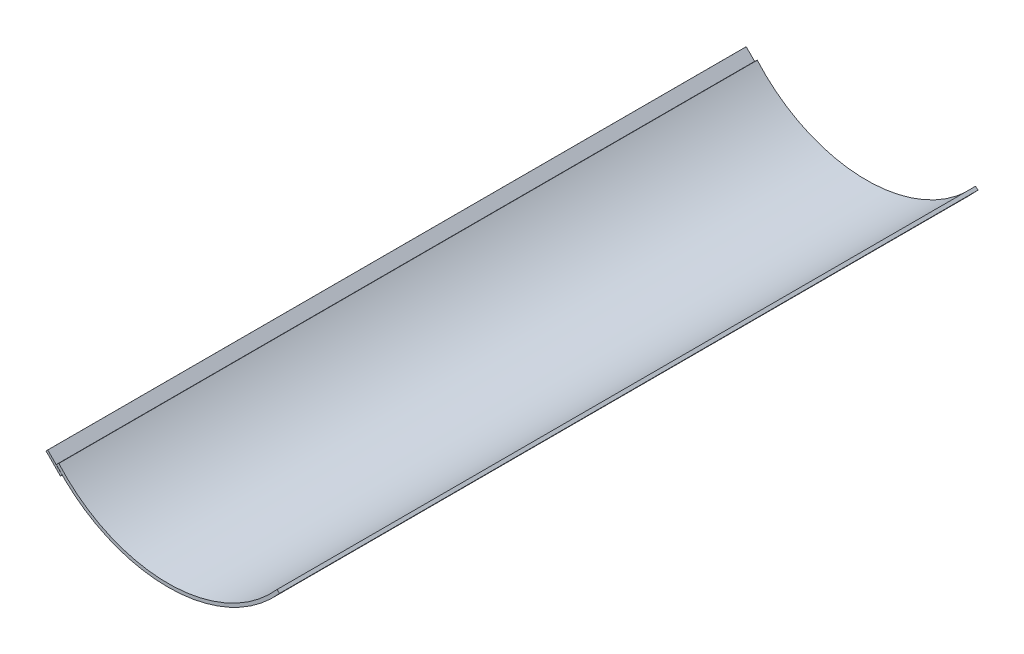
SolidWorks part; units mm, degrees
material "Q235A"
ref_plane "前视基准面" through (0, 0, 0) normal (0, 0, 1) x (1, 0, 0)
ref_plane "上视基准面" through (0, 0, 0) normal (0, 1, 0) x (1, 0, 0)
ref_plane "右视基准面" through (0, 0, 0) normal (1, 0, 0) x (0, 0, -1)
sketch "草图1" plane through (0, 0, 0) normal (0, 0, 1) x (1, 0, 0)
  line L0 (-132.8157, -117) -> (132.8157, -117) construction
  line L1 (0, 0) -> (0, 281.657) construction
  arc A0 (-132.8157, -117) -> (132.8157, -117) centre (0, 0) ccw
  dimension "D1" = 354
  dimension "D2" = 60
extrude "拉伸-薄壁1" add sketch "草图1" along normal mid plane 850 thin
sketch "草图2" plane through (0, 0, -425) normal (0, 0, -1) x (-1, 0, 0)
  line L0 (146.2589, -109.5186) -> (128.6772, -127.2917)
  line L1 (128.6772, -127.2917) -> (130.8099, -129.4015)
  line L2 (130.8099, -129.4015) -> (148.3917, -111.6285)
  line L3 (148.3917, -111.6285) -> (146.2589, -109.5186)
  line L5 (135.8171, -119.6441) -> (132.8157, -117) construction
  arc A0 (-135.8171, -119.6441) -> (135.8171, -119.6441) centre (0, 0) ccw construction
  dimension "D1" = 3
  dimension "D2" = 14.5
  dimension "D3" = 25
extrude "凸台-拉伸1" add sketch "草图2" against normal through all separate body
